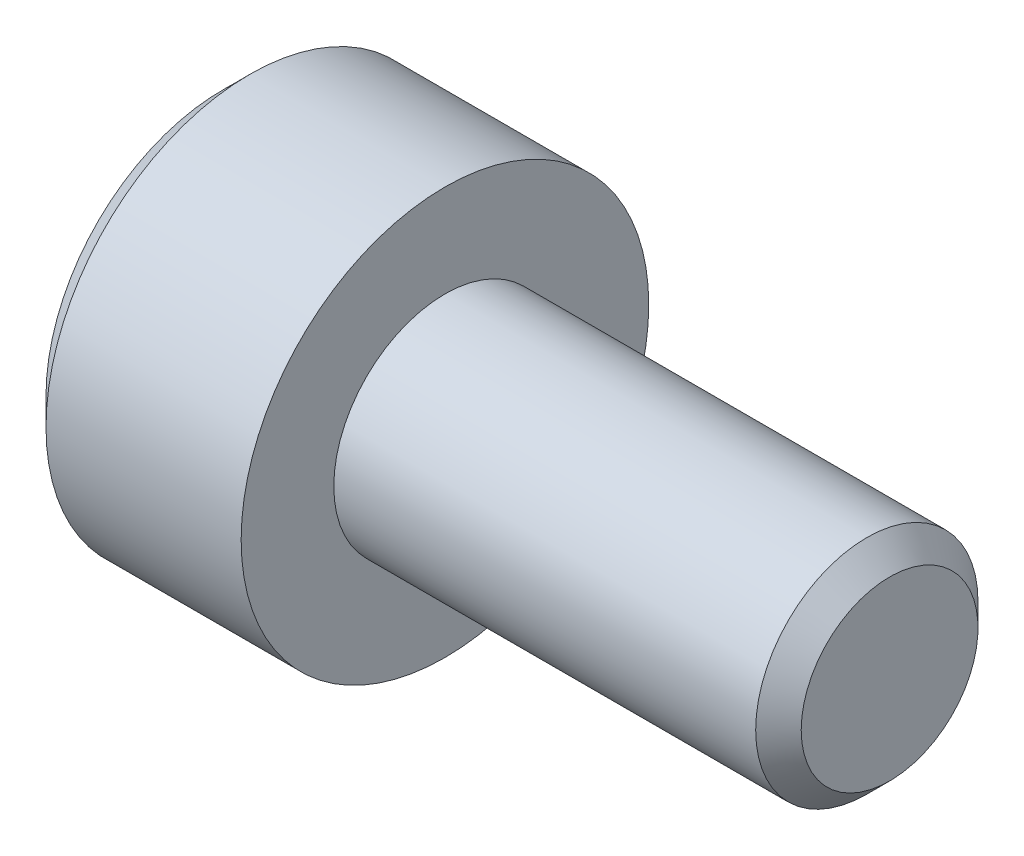
SolidWorks part; units mm, degrees
material "AISI 304"
ref_plane "Front Plane" through (0, 0, 0) normal (0, 0, 1) x (1, 0, 0)
ref_plane "Top Plane" through (0, 0, 0) normal (0, 1, 0) x (1, 0, 0)
ref_plane "Right Plane" through (0, 0, 0) normal (1, 0, 0) x (0, 0, -1)
sketch "Sketch1" plane through (0, 0, 0) normal (0, 0, 1) x (1, 0, 0)
  line L0 (-3, 0) -> (-3, 2.3833)
  line L1 (-3, 2.3833) -> (-2.6333, 2.75)
  line L2 (-2.6333, 2.75) -> (0, 2.75)
  line L3 (0, 2.75) -> (0, 1.5)
  line L4 (0, 1.5) -> (5.6928, 1.5)
  line L5 (5.6928, 1.5) -> (6, 1.1928)
  line L6 (6, 1.1928) -> (6, 0)
  line L7 (6, 0) -> (-3, 0)
  line L8 (6, 0) -> (-3, 0) construction
revolve "Revolve1" add sketch "Sketch1" angle 360 about L8
cosmetic thread "Cosmetic Thread1" parameters "D1"=5.468, "D2"=2.3857
sketch "Sketch2" plane through (0, 0, 0) normal (0, 0, 1) x (1, 0, 0)
  line L0 (-3, 0) -> (-3, 1.25)
  line L1 (-3, 1.25) -> (-1.5, 1.25)
  line L2 (-1.5, 1.25) -> (-1.1651, 0)
  line L3 (-1.1651, 0) -> (-3, 0)
  line L4 (-1.1651, 0) -> (-3, 0) construction
revolve "Cut-Revolve1" cut sketch "Sketch2" angle 360 about L4
ref_plane "Plane1" through (-3, 0, 0) normal (1, 0, 0) x (0, 0, -1)
sketch "Sketch3" plane through (-3, 0, 0) normal (1, 0, 0) x (0, 0, -1)
  line L0 (-1.25, 0.7217) -> (-1.25, -0.7217)
  line L1 (-1.25, -0.7217) -> (0, -1.4434)
  line L2 (0, -1.4434) -> (1.25, -0.7217)
  line L3 (1.25, -0.7217) -> (1.25, 0.7217)
  line L4 (1.25, 0.7217) -> (0, 1.4434)
  line L5 (0, 1.4434) -> (-1.25, 0.7217)
extrude "Cut-Extrude1" cut sketch "Sketch3" along normal blind 1.5
